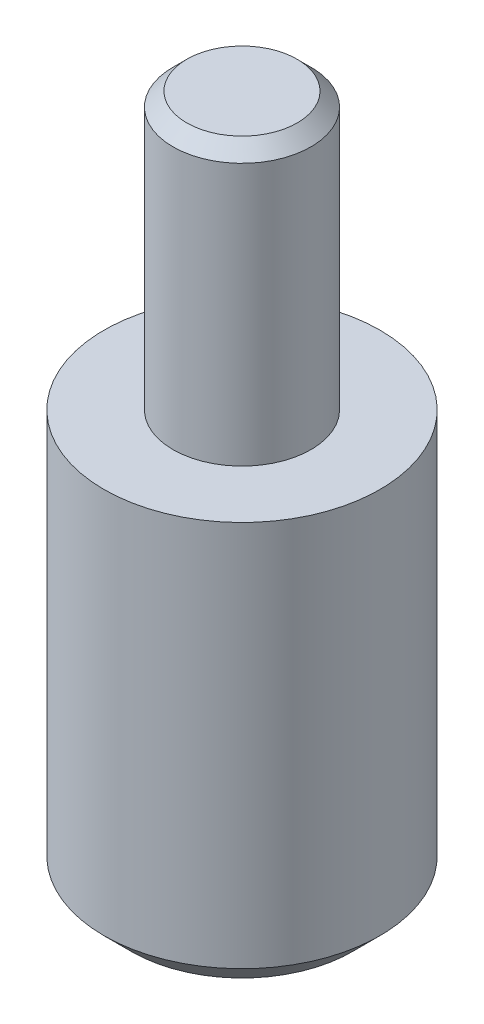
SolidWorks part; units mm, degrees
ref_plane "Front Plane" through (0, 0, 0) normal (0, 0, 1) x (1, 0, 0)
ref_plane "Top Plane" through (0, 0, 0) normal (0, 1, 0) x (1, 0, 0)
ref_plane "Right Plane" through (0, 0, 0) normal (1, 0, 0) x (0, 0, -1)
sketch "Sketch1" plane through (0, 0, 0) normal (0, 1, 0) x (1, 0, 0)
  circle A0 centre (0, 0) radius 10
  dimension "D1" = 20
extrude "Boss-Extrude1" add sketch "Sketch1" along normal blind 30
sketch "Sketch2" plane through (0, 30, 0) normal (0, 1, 0) x (1, 0, 0)
  circle A0 centre (0, 0) radius 5
  dimension "D1" = 10
extrude "Boss-Extrude2" add sketch "Sketch2" along normal blind 20
chamfer "Chamfer1" distance 2 angle 45 1 edges at (0, 0, 10)
chamfer "Chamfer2" distance 1 angle 45 1 edges at (0, 50, 5)
